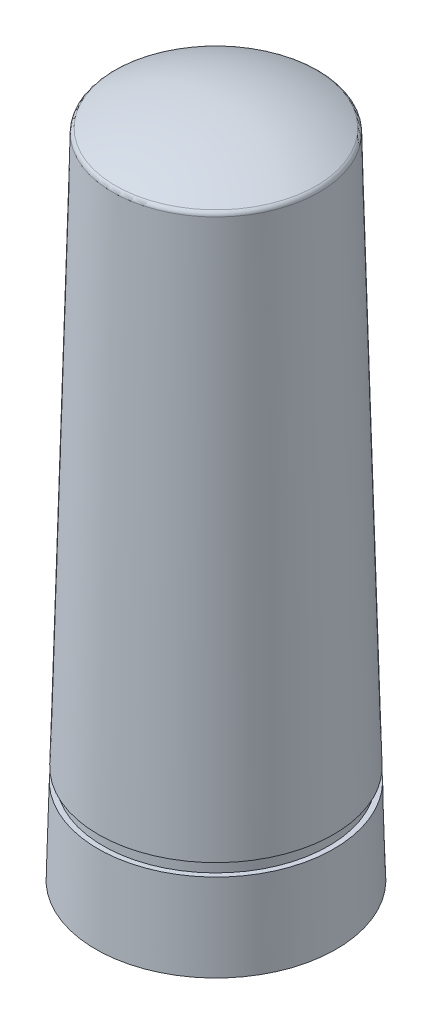
SolidWorks part; units mm, degrees
material "ABS"
ref_plane "Front Plane" through (0, 0, 0) normal (0, 0, 1) x (1, 0, 0)
ref_plane "Top Plane" through (0, 0, 0) normal (0, 1, 0) x (1, 0, 0)
ref_plane "Right Plane" through (0, 0, 0) normal (1, 0, 0) x (0, 0, -1)
sketch "Sketch1" plane through (0, 0, 0) normal (0, 0, 1) x (1, 0, 0)
  line L0 (0, 0) -> (0, 34.3143) construction
  line L1 (-4.9, 0) -> (-4.8075, 3.5)
  line L2 (0, 27.5) -> (3.345, 27.5) construction
  line L3 (-4.8075, 3.5) -> (-4.6, 3.5)
  line L4 (-4.6, 3.5) -> (-4.6, 4)
  line L5 (-4.6, 4) -> (-4.7943, 4)
  line L6 (-4.7943, 4) -> (-4.2032, 26.3797)
  line L7 (-4.9, 0) -> (-4, 0)
  line L8 (-4, 0) -> (-4, 1)
  line L9 (-4, 1) -> (-3.75, 1)
  line L10 (-3.25, 26.3797) -> (0, 26.3797)
  line L11 (0, 26.3797) -> (0, 27.5)
  line L12 (-3.75, 1) -> (-3.25, 26.3797)
  arc A0 (-4.091, 26.5541) -> (0, 27.5) centre (0, 18.18) cw
  arc A1 (-4.2032, 26.3797) -> (-4.091, 26.5541) centre (-4.0032, 26.3744) cw
  point P18 (-4.2, 26.5)
  dimension "D4" = 27.5
  dimension "D10" = 0.2
  dimension "D1" = 9.8
  dimension "D2" = 8.4
  dimension "D3" = 26.5
  dimension "D5" = 3.5
  dimension "D6" = 0.5
  dimension "D7" = 9.2
  dimension "D8" = 8
  dimension "D9" = 1
  dimension "D11" = 7.5
  dimension "D12" = 6.5
revolve "Revolve1" add sketch "Sketch1" angle 360 about L0
